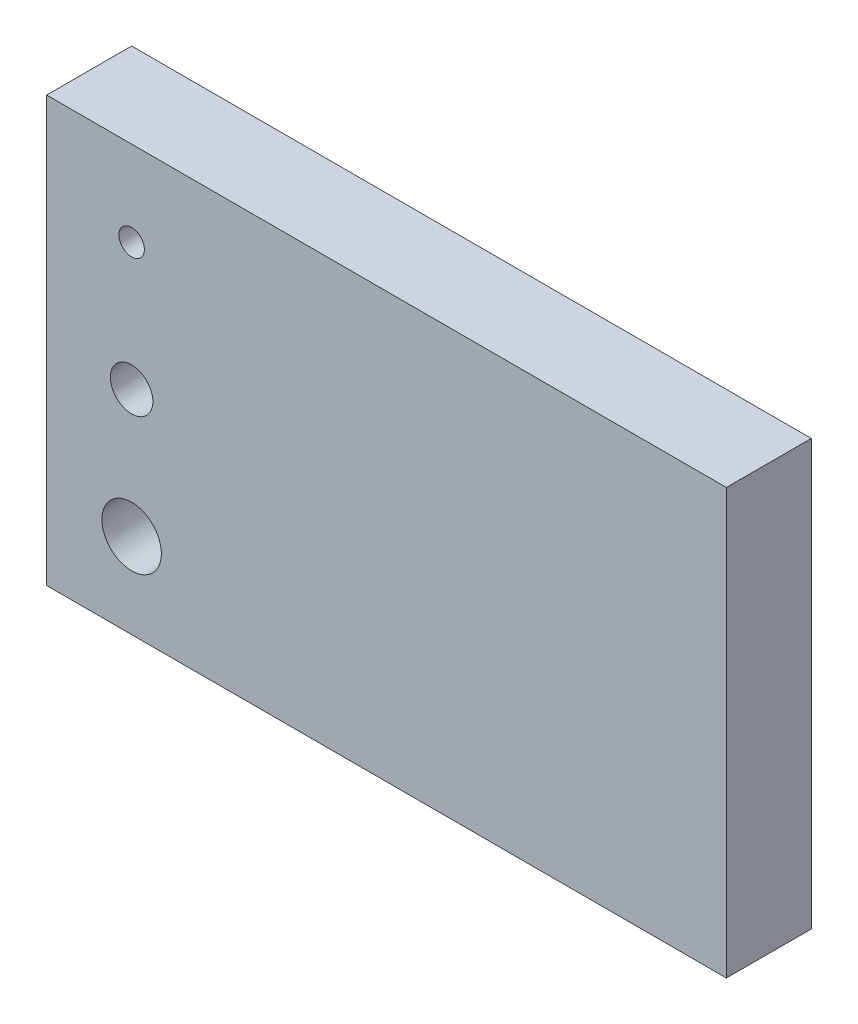
from build123d import *

# Parameters (mm, degrees)
SKETCH1_W           = 8
SKETCH1_H           = 6
BOSS_EXTRUDE1_DEPTH = 1
SKETCH2_R           = 0.15
SKETCH2_R_2         = 0.25
SKETCH2_R_3         = 0.35
CUT_EXTRUDE1_DEPTH  = 2
SKETCH3_W           = 8
SKETCH3_H           = 0.5
CUT_EXTRUDE2_DEPTH  = 7


with BuildPart() as part:
    # Sketch1 → Boss-Extrude1 (new body)
    with BuildSketch(Plane.XY):
        with Locations((4, -3)):
            Rectangle(SKETCH1_W, SKETCH1_H)
    extrude(amount=BOSS_EXTRUDE1_DEPTH)

    # Sketch2 → Cut-Extrude1 (cut)
    with BuildSketch(Plane.XY.offset(1)):
        with Locations((1, -1.5)):
            Circle(SKETCH2_R)
        with Locations((1, -3)):
            Circle(SKETCH2_R_2)
        with Locations((1, -4.5)):
            Circle(SKETCH2_R_3)
    extrude(amount=-CUT_EXTRUDE1_DEPTH, mode=Mode.SUBTRACT)

    # Sketch3 → Cut-Extrude2 (cut)
    with BuildSketch(Plane.XY.offset(1)):
        with Locations((4, -0.25)):
            Rectangle(SKETCH3_W, SKETCH3_H)
        with Locations((4, -5.75)):
            Rectangle(SKETCH3_W, SKETCH3_H)
    extrude(amount=-CUT_EXTRUDE2_DEPTH, mode=Mode.SUBTRACT)


solid = part.part
